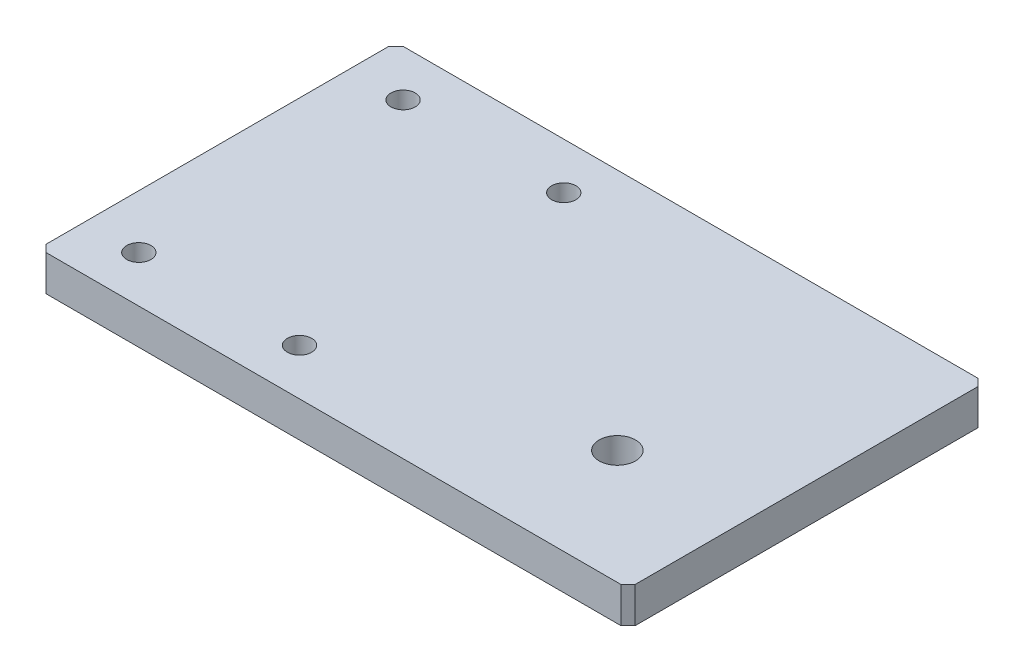
SolidWorks part; units mm, degrees
material "普通碳钢"
ref_plane "前视基准面" through (0, 0, 0) normal (0, 0, 1) x (1, 0, 0)
ref_plane "上视基准面" through (0, 0, 0) normal (0, 1, 0) x (1, 0, 0)
ref_plane "右视基准面" through (0, 0, 0) normal (1, 0, 0) x (0, 0, -1)
sketch "草图1" plane through (0, 0, 0) normal (0, 1, 0) x (1, 0, 0)
  line L1 (-82.5, 50) -> (82.5, 50)
  line L2 (-82.5, 50) -> (-82.5, -50)
  line L3 (-82.5, -50) -> (82.5, -50)
  line L4 (82.5, 50) -> (82.5, -50)
  line L5 (-82.5, 50) -> (82.5, -50) construction
  line L6 (-82.5, -50) -> (82.5, 50) construction
  point P0 (0, 0)
  dimension "D1" = 165
  dimension "D2" = 100
extrude "凸台-拉伸1" add sketch "草图1" along normal blind 10
hole_wizard "M8 螺纹孔1" positions "草图3" profile "草图2" tap size "M8" standard "GB"
sketch "草图3" plane through (0, 10, 0) normal (0, 1, 0) x (1, 0, 0)
  line L0 (-82.5, 0) -> (82.5, 0) construction
  line L1 (-82.5, 50) -> (-82.5, -50) construction
  line L2 (82.5, -50) -> (82.5, 50) construction
  point P0 (-67.5, 37)
  point P2 (-22.5, 37)
  point P15 (-22.5, -37)
  point P16 (-67.5, -37)
  dimension "D1" = 15
  dimension "D2" = 45
  dimension "D3" = 74
sketch "草图2" plane through (-67.5, 10, -37) normal (1, 0, 0) x (0, 0, 1)
  line L0 (0, 0) -> (0, 18.2929)
  line L1 (0, 18.2929) -> (3.4, 16.25)
  line L2 (3.4, 16.25) -> (3.4, 0)
  line L5 (3.4, 0) -> (0, 0)
  line L10 (0, 18.2929) -> (-3.4, 16.25) construction
  line L11 (0, -6.35) -> (0, 107.95) construction
  dimension "螺纹孔钻头直径" = 6.8
  dimension "螺纹孔钻头深度" = 16.25
  dimension "导头角度" = 118
cosmetic thread "孔螺蚊线1" parameters "D1"=10, "D2"=8
cosmetic thread "孔螺蚊线2" parameters "D1"=10, "D2"=8
cosmetic thread "孔螺蚊线3" parameters "D1"=10, "D2"=8
cosmetic thread "孔螺蚊线4" parameters "D1"=10, "D2"=8
hole_wizard "M12 螺纹孔1" positions "草图5" profile "草图4" tap size "M12" standard "GB"
sketch "草图5" plane through (0, 10, 0) normal (0, 1, 0) x (1, 0, 0)
  line L0 (-82.5, -50) -> (82.5, -50) construction
  line L1 (82.5, -50) -> (82.5, 50) construction
  point P0 (47.5, -18)
  dimension "D1" = 32
  dimension "D2" = 35
sketch "草图4" plane through (47.5, 10, 18) normal (1, 0, 0) x (0, 0, 1)
  line L0 (0, 0) -> (0, 35.8144)
  line L1 (0, 35.8144) -> (5.1, 32.75)
  line L2 (5.1, 32.75) -> (5.1, 0)
  line L5 (5.1, 0) -> (0, 0)
  line L10 (0, 35.8144) -> (-5.1, 32.75) construction
  line L11 (0, -6.35) -> (0, 107.95) construction
  dimension "螺纹孔钻头直径" = 10.2
  dimension "螺纹孔钻头深度" = 32.75
  dimension "导头角度" = 118
cosmetic thread "孔螺蚊线5" parameters "D1"=10, "D2"=12
chamfer "倒角1" distance 2 angle 45 4 edges at (82.5, 5, -50) (-82.5, 5, -50) (-82.5, 5, 50) (82.5, 5, 50)
